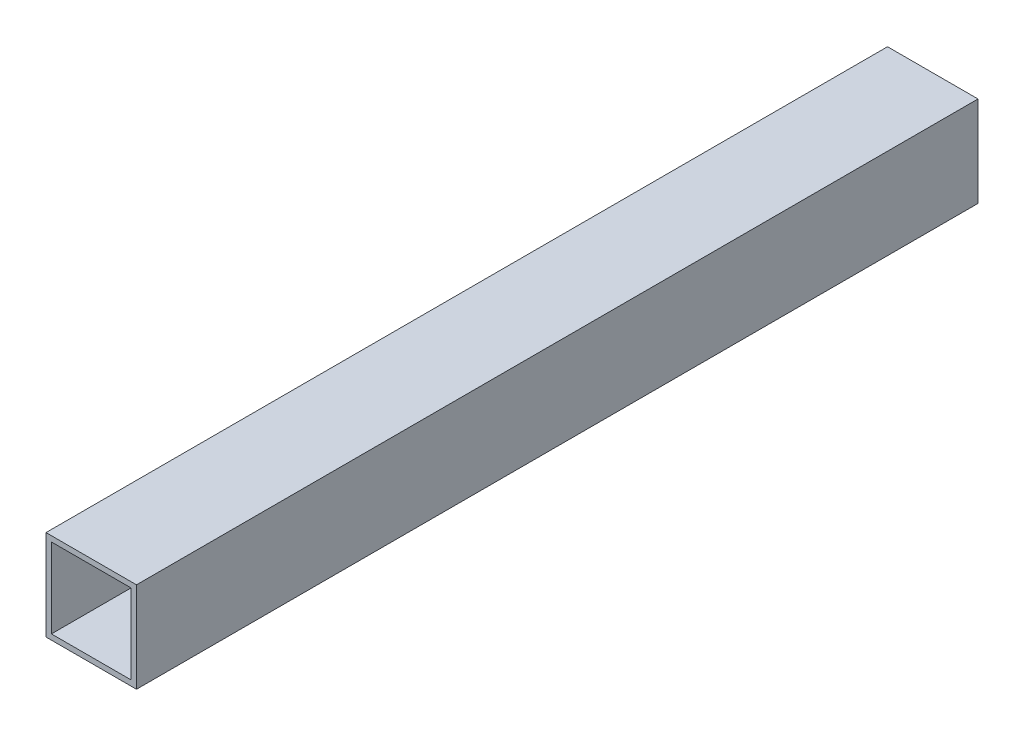
SolidWorks part; units mm, degrees
ref_plane "前视基准面" through (0, 0, 0) normal (0, 0, 1) x (1, 0, 0)
ref_plane "上视基准面" through (0, 0, 0) normal (0, 1, 0) x (1, 0, 0)
ref_plane "右视基准面" through (0, 0, 0) normal (1, 0, 0) x (0, 0, -1)
sketch "草图1" plane through (0, 0, 0) normal (0, 0, 1) x (1, 0, 0)
  line L0 (0, 0) -> (0, 50)
  line L1 (0, 50) -> (50, 50)
  line L2 (50, 50) -> (50, 0)
  line L3 (50, 0) -> (0, 0)
  line L4 (3, 3) -> (3, 47)
  line L5 (3, 47) -> (47, 47)
  line L6 (47, 47) -> (47, 3)
  line L7 (47, 3) -> (3, 3)
  dimension "D1" = 3
extrude "凸台-拉伸1" add sketch "草图1" along normal blind 465
